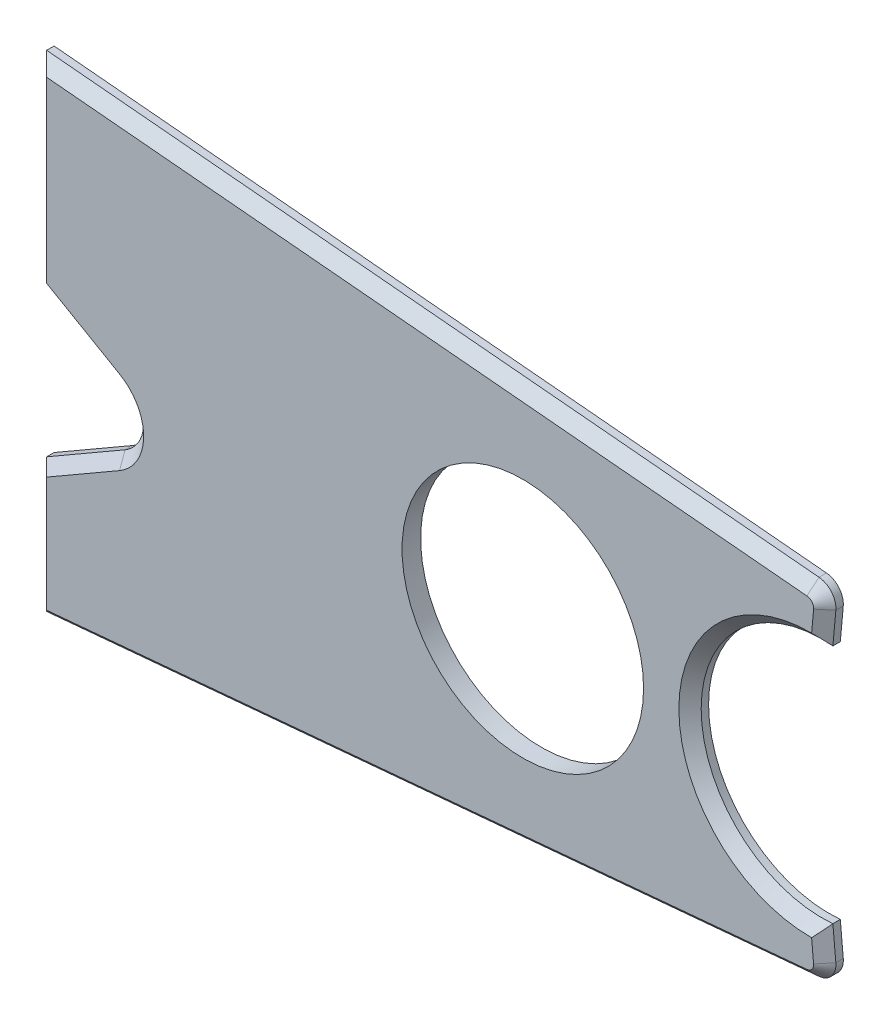
from build123d import *

# Parameters (mm, degrees)
SKETCH1_R           = 65
BOSS_EXTRUDE1_DEPTH = 10
CHAMFER1_SIZE       = 6


with BuildPart() as part:
    # Sketch1 → Boss-Extrude1 (new body)
    with BuildSketch(Plane.XY):
        with BuildLine():
            Line((-262.3, 130.8), (-262.3, 24.7))
            Line((-262.3, 24.7), (-220.073481324, 0.320508076))
            ThreePointArc((-220.073481324, 0.320508076), (-210.073481324, -17), (-220.073481324, -34.320508076))
            Line((-220.073481324, -34.320508076), (-262.3, -58.7))
            Line((-262.3, -58.7), (-262.3, -130.8))
            Line((-262.3, -130.8), (153.441030377, -93.022753927))
            ThreePointArc((153.441030377, -93.022753927), (160.218033303, -89.465947057), (162.495055771, -82.158840075))
            Line((162.495055771, -82.158840075), (160.91140277, -64.73063662))
            ThreePointArc((160.91140277, -64.73063662), (90, 0), (160.91140277, 64.73063662))
            Line((160.91140277, 64.73063662), (162.495055771, 82.158840075))
            ThreePointArc((162.495055771, 82.158840075), (160.218033303, 89.465947057), (153.441030377, 93.022753927))
            Line((153.441030377, 93.022753927), (-262.3, 130.8))
        make_face()
        Circle(SKETCH1_R, mode=Mode.SUBTRACT)
    extrude(amount=BOSS_EXTRUDE1_DEPTH)

    # Chamfer1
    chamfer1_edges = [part.edges().sort_by_distance(p)[0] for p in [
        (160.218033303, -89.465947057, 10),
        (161.703229271, -73.444738348, 10),
        (90, 0, 10),
        (161.703229271, 73.444738348, 10),
        (160.218033303, 89.465947057, 10),
        (-54.429484811, 111.911376963, 10),
        (-262.3, 77.75, 10),
        (-241.186740662, 12.510254038, 10),
        (-210.073481324, -17, 10),
        (-241.186740662, -46.510254038, 10),
        (-262.3, -94.75, 10),
        (-54.429484811, -111.911376963, 10),
    ]]
    chamfer(chamfer1_edges, length=CHAMFER1_SIZE)


solid = part.part
